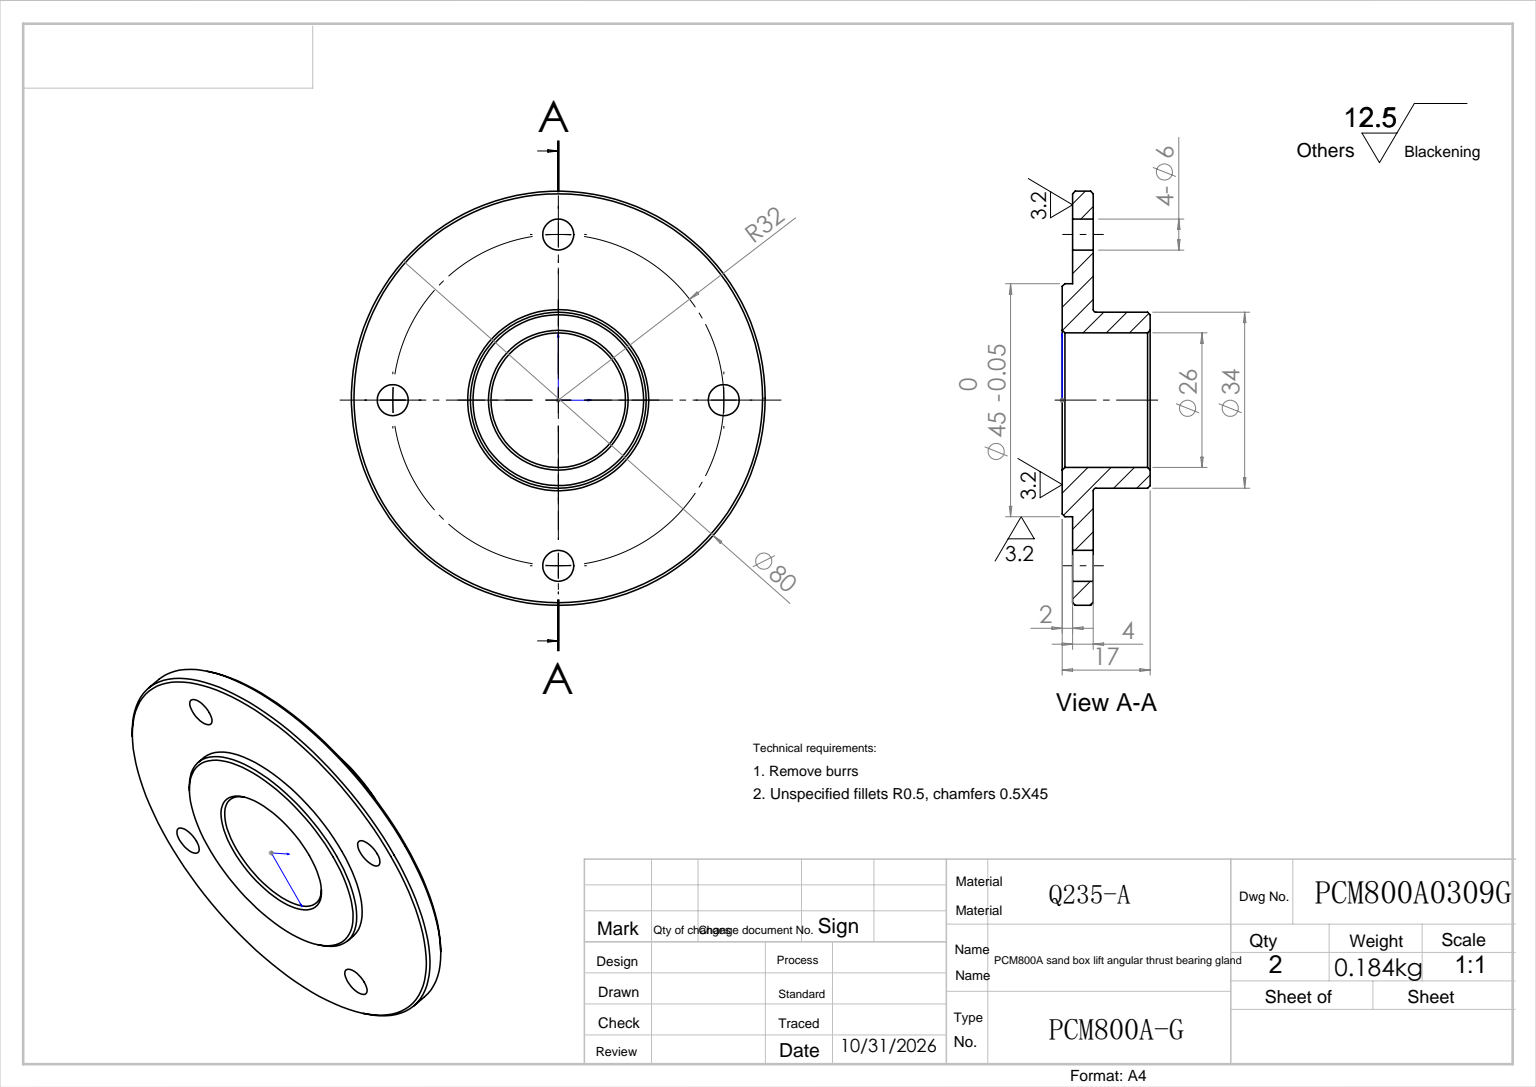
from build123d import *

# Parameters (mm, degrees)
SKETCH_1_R          = 22.5
SKETCH_1_R_2        = 13
EXTRUDE_1_DEPTH     = 2
SKETCH_2_R          = 40
SKETCH_2_R_2        = 13
EXTRUDE_2_DEPTH     = 4
SKETCH_3_R          = 17
SKETCH_3_R_2        = 13
EXTRUDE_3_DEPTH     = 11
CHAMFER_1_SIZE      = 0.5
FILLET_1_R          = 0.5
SKETCH_4_R          = 3
CUT_EXTRUDE_1_DEPTH = 58.888606929


with BuildPart() as part:
    # 草图1 → 拉伸1 (new body)
    with BuildSketch(Plane.XY):
        Circle(SKETCH_1_R)
        Circle(SKETCH_1_R_2, mode=Mode.SUBTRACT)
    extrude(amount=EXTRUDE_1_DEPTH)

    # 草图2 → 拉伸2 (add)
    with BuildSketch(Plane.XY.offset(2)):
        with Locations((0, 0.374383119)):
            Circle(SKETCH_2_R)
        Circle(SKETCH_2_R_2, mode=Mode.SUBTRACT)
    extrude(amount=EXTRUDE_2_DEPTH)

    # 草图3 → 拉伸3 (add)
    with BuildSketch(Plane.XY.offset(6)):
        Circle(SKETCH_3_R)
        Circle(SKETCH_3_R_2, mode=Mode.SUBTRACT)
    extrude(amount=EXTRUDE_3_DEPTH)

    # 倒角1
    chamfer_1_edges = [part.edges().sort_by_distance(p)[0] for p in [
        (-40, 0.374383119, 2),
        (-17, 0, 17),
        (-13, 0, 17),
        (-22.5, 0, 0),
        (-13, 0, 0),
        (-40, 0.374383119, 6),
    ]]
    chamfer(chamfer_1_edges, length=CHAMFER_1_SIZE)

    # 圆角1
    fillet_1_edges = [part.edges().sort_by_distance(p)[0] for p in [
        (-17, 0, 6),
    ]]
    fillet(fillet_1_edges, radius=FILLET_1_R)

    # 草图4 → 切除-拉伸1 (cut, through all)
    with BuildSketch(Plane.XY.offset(6)):
        with Locations((0, 32)):
            Circle(SKETCH_4_R)
        with Locations((-32, 0)):
            Circle(SKETCH_4_R)
        with Locations((0, -32)):
            Circle(SKETCH_4_R)
        with Locations((32, 0)):
            Circle(SKETCH_4_R)
    extrude(amount=-CUT_EXTRUDE_1_DEPTH, mode=Mode.SUBTRACT)


solid = part.part
